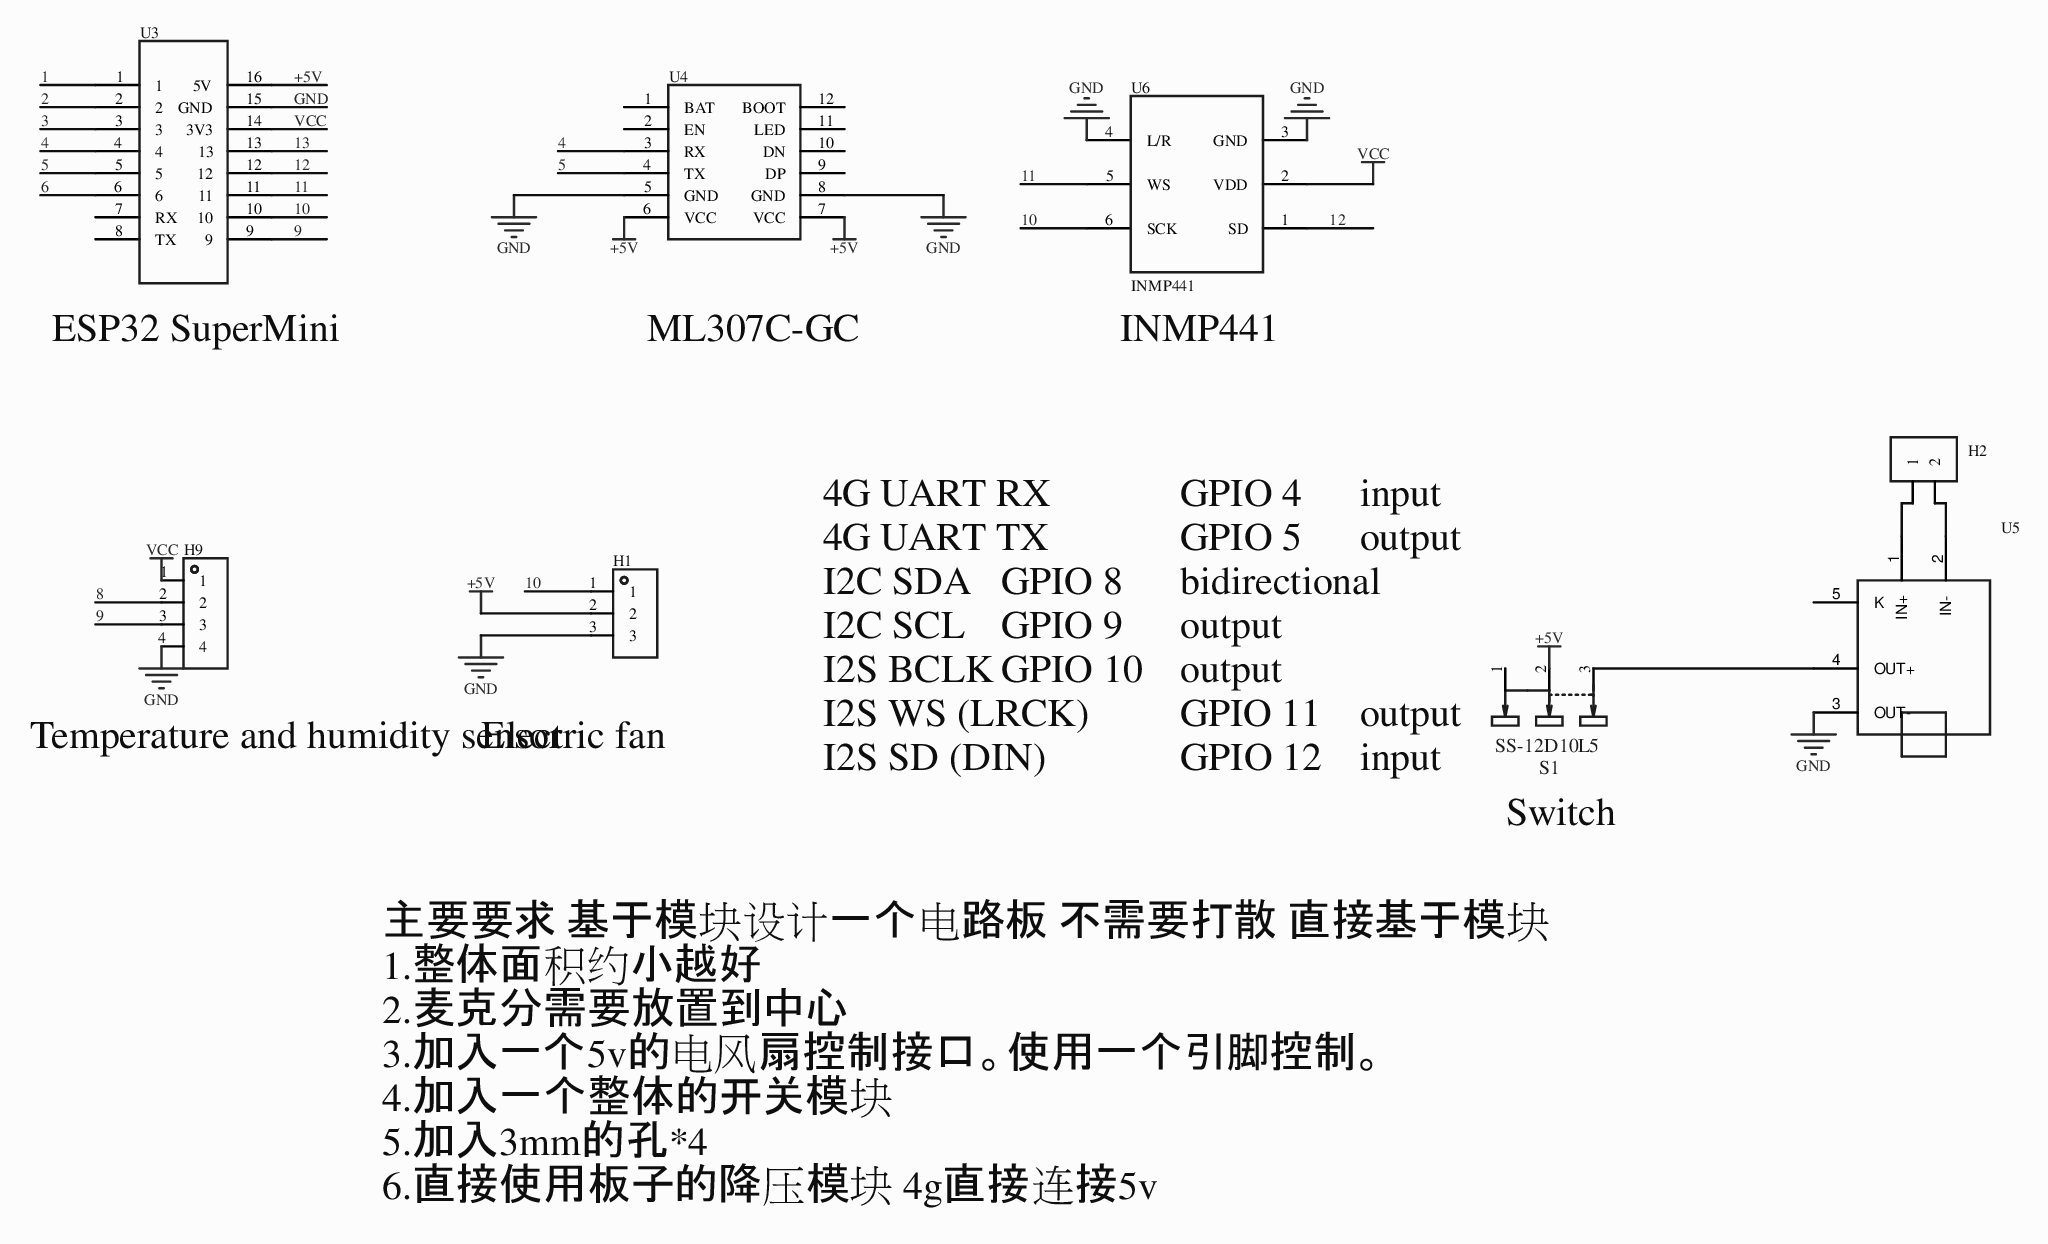
[diagram p0: MISC79010-3.schdoc]
# Altium project MISC79010-2.PrjPcb
1 sheet, 8 parts. Net scope: global (net labels, ports and power ports of the same name join across sheets).
Board file: MISC79010.pcbdoc

## Sheet MISC79010-3.schdoc
size 297 x 209 mm; Version: V1.0; @Project Name: MISC79010; @Page Count: 1; @Update Date: 2026-05-20; @Create Date: 2026-05-20; @Schematic Name: MISC79010; @Page No: 1; @Create Time: 23:22:16; @Update Time: 17:32:40; @Board Name: MISC79010

### Parts
H1  (no value)  [HDR-TH_3P-P2.54-V-M]
H2  (no value)  [HDR-TH_2P-P2.54-V-F]
H9  (no value)  [HDR-TH_4P-P2.54-V-F]
S1  SS-12D10L5  [SS-12D10L5]
U3  (no value)  [【封装Supermini】]
U4  (no value)  [ML307C-GC核心板]
U5  (no value)  [5V2A充放电一体模块]
U6  INMP441  [INMP441]

### Nets
+5V: H1.2 S1.2 U3.16(5V) U4.6(VCC) U4.7(VCC)
GND: H1.3 H9.4 U3.15(GND) U4.5(GND) U4.8(GND) U5.3(OUT-) U6.3(GND) U6.4(L/R)
VCC: H9.1 U3.14(3V3) U6.2(VDD)
1: U3.1
2: U3.2
3: U3.3
4: U3.4 U4.3(RX)
5: U3.5 U4.4(TX)
6: U3.6
8: H9.2
9: H9.3 U3.9
10: H1.1 U3.10 U6.6(SCK)
11: U3.11 U6.5(WS)
12: U3.12 U6.1(SD)
13: U3.13
NetH2_1: H2.1 U5.1(IN+)
NetH2_2: H2.2 U5.2(IN-)
NetS1_3: S1.3 U5.4(OUT+)

Not connected (* = marked no-connect by the designer): S1 1; U3 7(RX) 8(TX); U4 1(BAT) 2(EN) 9(DP) 10(DN) 11(LED) 12(BOOT); U5 5(K)

### Notes on the sheet
- (near U3) ESP32 SuperMini
- ML307C-GC
- (near U6) INMP441
- 4G UART RX	GPIO 4	input
  4G UART TX	GPIO 5	output
  I2C SDA	GPIO 8	bidirectional
  I2C SCL	GPIO 9	output
  I2S BCLK	GPIO 10	output
  I2S WS (LRCK)	GPIO 11	output
  I2S SD (DIN)	GPIO 12	input
- Temperature and humidity sensor
- (near H1) Electric fan
- Switch
- 主要要求 基于模块设计一个电路板 不需要打散 直接基于模块
  1.整体面积约小越好
  2.麦克分需要放置到中心
  3.加入一个5v的电风扇控制接口。使用一个引脚控制。
  4.加入一个整体的开关模块
  5.加入3mm的孔*4
  6.直接使用板子的降压模块 4g直接连接5v

### Library data of the parts
H1 = HDR-M_2.54_1x3P: AddInBom: yes; ModelId: bb473b6d38ff42a99216a4fcdbdcc4cb0819f05c4eef4c71ace90d822a990e87; ModelName: HDR-TH_3P-P2.54-M-LI-1X3P; ModelTransform: 300.03877,100,0,0,0,0,0,0,-118.11; Symbol: HDR-M_2.54_1x3P; Device: HDR-M_2.54_1x3P; ConvertToPcb: yes; FootprintName: HDR-TH_3P-P2.54-V-M; SupplierPart: C2937625; Supplier Footprint: 插件
H2 = HDR-F_2.54_1x2P: Symbol: Header-Female-2.54_1x2; ConvertToPcb: yes; ModelId: a9450ef445564560a104363b9aacde4e; ModelName: HDR-TH_2P-P2.54-F-LI-1X2P; ModelTransform: 215.7476,98.425,0,0,0,0,0,0,-129.921; Device: HDR-F_2.54_1x2P; AddInBom: yes; SupplierPart: C49661; Supplier Footprint: 插件; FootprintName: HDR-TH_2P-P2.54-V-F
H9 = HDR-F_2.54_1x4P: Symbol: 2.54-1*4P female; ConvertToPcb: yes; ModelId: d187812051054f85879fcaa51a310d8e0819f05c4eef4c71ace90d822a990e87; ModelTransform: 419.6842,98.464,0,0,0,0,0,0,-118.11; Device: HDR-F_2.54_1x4P; AddInBom: yes; SupplierPart: C2718488; Supplier Footprint: 插件; FootprintName: HDR-TH_4P-P2.54-V-F; ModelName: HDR-TH_4P-P2.54-V-F
S1 = SS-12D10L5: AddInBom: yes; ModelId: e87b8ea3587d4b928695d6d9193d4eb2dc1a613412b64707ae36f77da95ce4a2; ModelTransform: 511.8099971175413,267.7160060014839,673.22703,0,0,0,0,0,-255.90551; Symbol: SS-12D10L5; Device: SS-12D10L5; ConvertToPcb: yes; Value: SS-12D10L5; FootprintName: SS-12D10L5; ModelName: SS-12D10L5
U3 = ESP32 SuperMini: AddInBom: yes; Symbol: ESP32 SuperMini; Device: ESP32 SuperMini; ConvertToPcb: yes; FootprintName: [Footprint Supermini]
U4 = ML307C-GC核心板: Symbol: ML307C-GC core board; AddInBom: yes; Device: ML307C-GC core board; FootprintName: ML307C-GC core board; ConvertToPcb: yes
U5 = 5V2A充放电一体模块: Symbol: 5V2A charge-discharge integrated module; AddInBom: yes; ModelId: 8f53618676814c9da935bcb72554571c44738c407a1041ee8aff7ec589a23399; ModelName: 3D_CKCS charging module; ModelTransform: 786.4,1038.51,175.24,180,0,0,0,-7.87,0; Device: 5V2A charge-discharge integrated module; ConvertToPcb: yes; FootprintName: 5V2A charge-discharge integrated module
U6 = INMP441: AddInBom: yes; Symbol: INMP441; Device: INMP441; ConvertToPcb: yes; FootprintName: INMP441